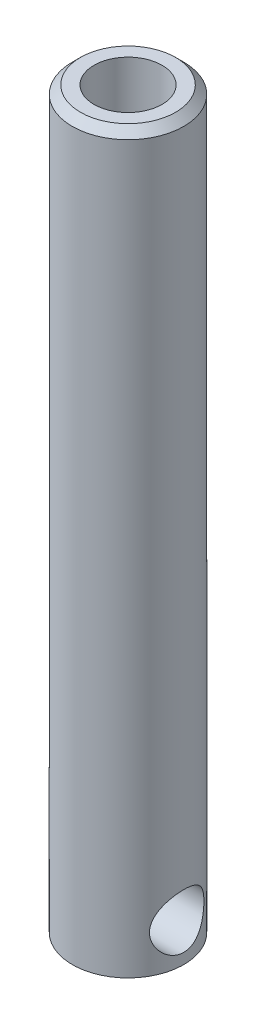
SolidWorks part; units mm, degrees
ref_plane "Front Plane" through (0, 0, 0) normal (0, 0, 1) x (1, 0, 0)
ref_plane "Top Plane" through (0, 0, 0) normal (0, 1, 0) x (1, 0, 0)
ref_plane "Right Plane" through (0, 0, 0) normal (1, 0, 0) x (0, 0, -1)
sketch "Sketch1" plane through (0, 0, 0) normal (0, 1, 0) x (1, 0, 0)
  circle A0 centre (0, 0) radius 205
  circle A1 centre (0, 0) radius 125
  dimension "D1" = 410
  dimension "D2" = 250
extrude "Boss-Extrude1" add sketch "Sketch1" along normal blind 2300
sketch "Sketch2" plane through (0, 0, 0) normal (0, -1, 0) x (1, 0, 0)
  circle A0 centre (0, 0) radius 205
  dimension "D1" = 410
extrude "Boss-Extrude2" add sketch "Sketch2" along normal blind 400
sketch "Sketch3" plane through (0, 0, 0) normal (1, 0, 0) x (0, 0, -1)
  line L0 (0, 225.5) -> (0, -225.5) construction
  circle A0 centre (0, -260.8437) radius 100
  dimension "D1" = 200
extrude "Cut-Extrude1" cut sketch "Sketch3" against normal blind 4000 and the other way blind 5000
chamfer "Chamfer1" distance 30 angle 45 1 edges at (0, 2300, 205)
